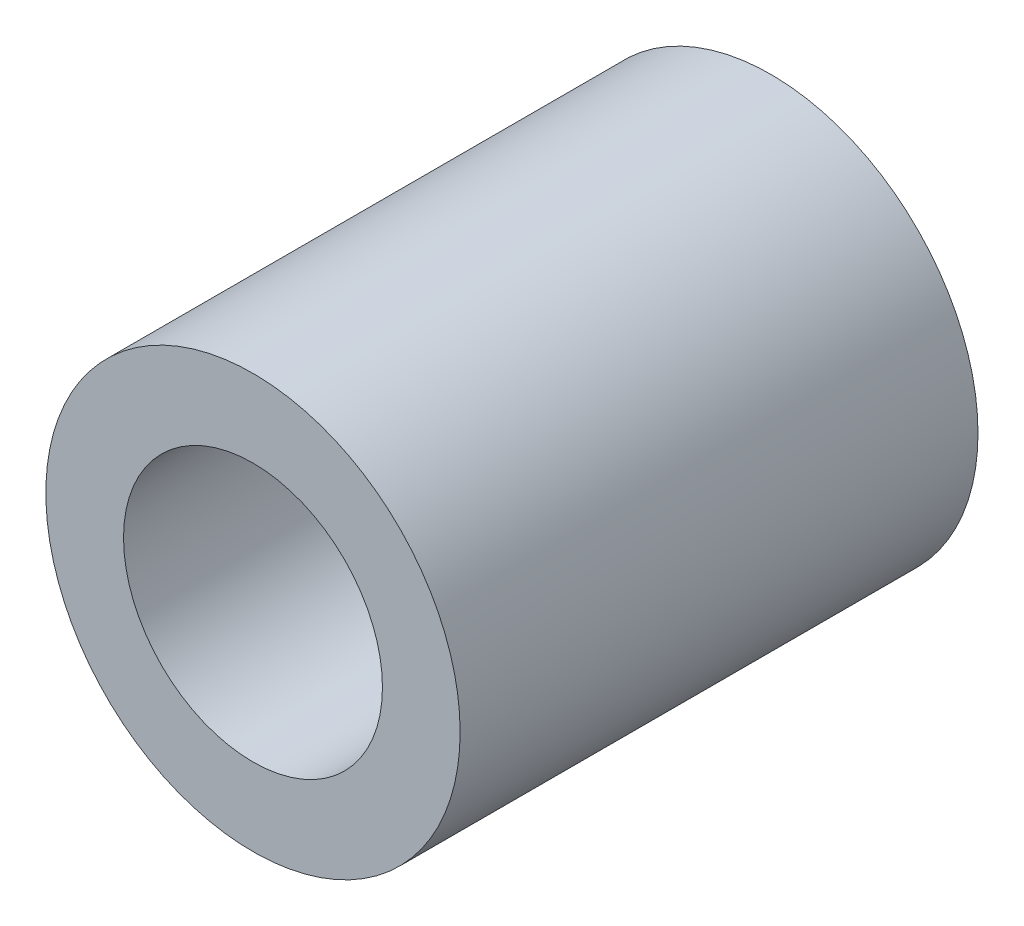
SolidWorks part; units mm, degrees
ref_plane "前视基准面" through (0, 0, 0) normal (0, 0, 1) x (1, 0, 0)
ref_plane "上视基准面" through (0, 0, 0) normal (0, 1, 0) x (1, 0, 0)
ref_plane "右视基准面" through (0, 0, 0) normal (1, 0, 0) x (0, 0, -1)
sketch "草图1" plane through (0, 0, 0) normal (0, 0, 1) x (1, 0, 0)
  circle A0 centre (0, 0) radius 20
  circle A1 centre (0, 0) radius 12.5
  dimension "D1" = 40
  dimension "D2" = 25
extrude "凸台-拉伸1" add sketch "草图1" along normal mid plane 50
